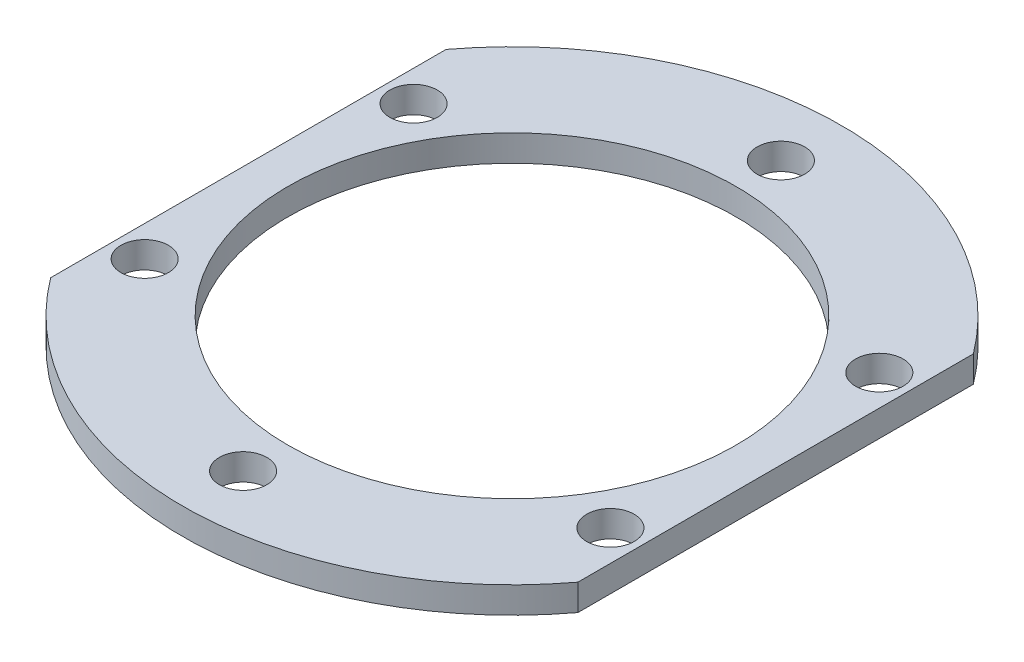
from build123d import *

# Parameters (mm, degrees)
SKETCH1_R           = 62.5
SKETCH1_R_2         = 42.5
BOSS_EXTRUDE1_DEPTH = 5
SKETCH2_R           = 4.5
CUT_EXTRUDE1_DEPTH  = 10
SKETCH3_OUTSIDE_W   = 162.37
SKETCH3_OUTSIDE_H   = 162.37
SKETCH3_OUTSIDE_W_2 = 100
SKETCH3_OUTSIDE_H_2 = 143.531180288
CUT_EXTRUDE2_DEPTH  = 10


with BuildPart() as part:
    # Sketch1 → Boss-Extrude1 (new body)
    with BuildSketch(Plane(origin=(0, 0, 0), x_dir=(1, 0, 0), z_dir=(0, 1, 0))):
        with Locations(Location((0, 0, 0), (0, 0, 270))):
            Circle(SKETCH1_R)
        with Locations(Location((0, 0, 0), (0, 0, 270))):
            Circle(SKETCH1_R_2, mode=Mode.SUBTRACT)
    extrude(amount=BOSS_EXTRUDE1_DEPTH)

    # Sketch2 → Cut-Extrude1 (cut)
    with BuildSketch(Plane(origin=(0, 5, 0), x_dir=(1, 0, 0), z_dir=(0, 1, 0))):
        with Locations(Location((0, 51, 0), (0, 0, 270))):
            Circle(SKETCH2_R)
        with Locations(Location((44.167295593, 25.5, 0), (0, 0, 270))):
            Circle(SKETCH2_R)
        with Locations(Location((44.167295593, -25.5, 0), (0, 0, 270))):
            Circle(SKETCH2_R)
        with Locations(Location((0, -51, 0), (0, 0, 270))):
            Circle(SKETCH2_R)
        with Locations(Location((-44.167295593, -25.5, 0), (0, 0, 270))):
            Circle(SKETCH2_R)
        with Locations(Location((-44.167295593, 25.5, 0), (0, 0, 270))):
            Circle(SKETCH2_R)
    extrude(amount=-CUT_EXTRUDE1_DEPTH, mode=Mode.SUBTRACT)

    # Sketch3 outside → Cut-Extrude2 (cut)
    with BuildSketch(Plane(origin=(0, 5, 0), x_dir=(1, 0, 0), z_dir=(0, 1, 0))):
        Rectangle(SKETCH3_OUTSIDE_W, SKETCH3_OUTSIDE_H)
        Rectangle(SKETCH3_OUTSIDE_W_2, SKETCH3_OUTSIDE_H_2, mode=Mode.SUBTRACT)
    extrude(amount=-CUT_EXTRUDE2_DEPTH, mode=Mode.SUBTRACT)


solid = part.part
